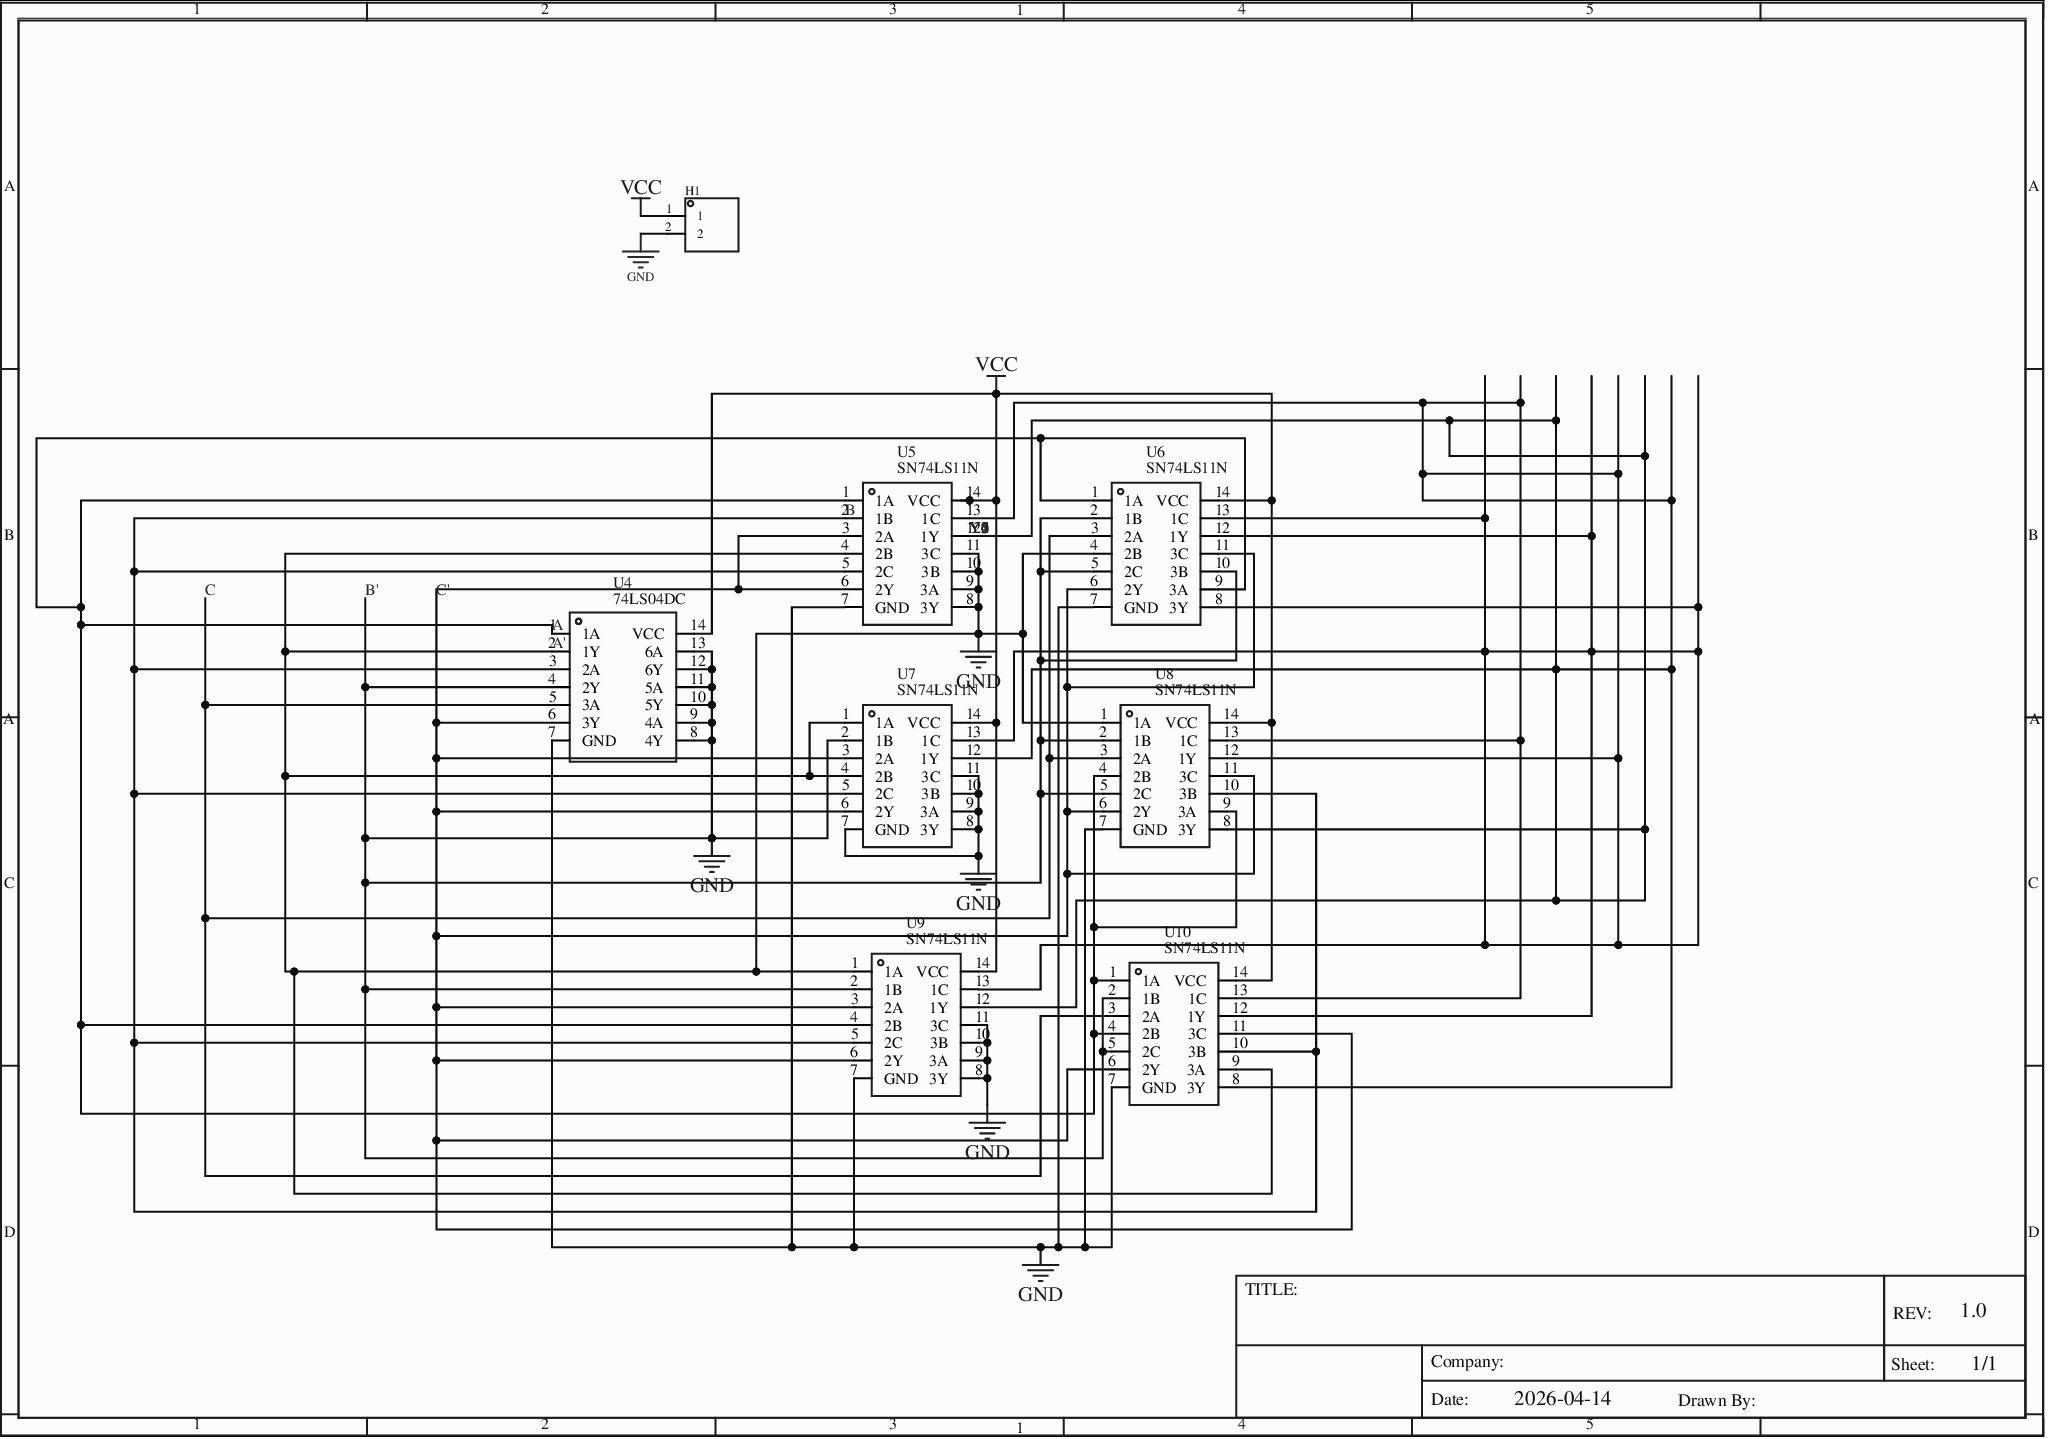
[diagram p0: MISC52068-3.schdoc]
# Altium project MISC52068-2.PrjPcb
3 sheets, 29 parts. Net scope: global (net labels, ports and power ports of the same name join across sheets).
Board file: MISC52068.pcbdoc
Sheets:
  MISC52068-3.schdoc
  MISC52068-4.schdoc
  MISC52068-5.schdoc

## Sheet MISC52068-3.schdoc
size 292 x 205 mm; Name: MISC52068; @Project Name: MISC52068; REV: 1.0; Date: 2026-04-14; Sheet: 1/1; Manufacturer Part: ?

### Parts
H1  (no value)  [HDR-TH_2P-P2.54-V-M-1]
U4  74LS04DC  [CDIP-14_L20.0-W6.8-P2.54-LS7.8-BL]
U5  SN74LS11N  [PDIP-14_L19.3-W6.4-P2.54-LS7.9-BL-1]
U6  SN74LS11N  [PDIP-14_L19.3-W6.4-P2.54-LS7.9-BL-1]
U7  SN74LS11N  [PDIP-14_L19.3-W6.4-P2.54-LS7.9-BL-1]
U8  SN74LS11N  [PDIP-14_L19.3-W6.4-P2.54-LS7.9-BL-1]
U9  SN74LS11N  [PDIP-14_L19.3-W6.4-P2.54-LS7.9-BL-1]
U10  SN74LS11N  [PDIP-14_L19.3-W6.4-P2.54-LS7.9-BL-1]

### Nets
A': H1.2 U4.2(1Y) U4.4(2Y) U4.7(GND) U4.8(4Y) U4.9(4A) U4.10(5Y) U4.11(5A) U4.12(6Y) U4.13(6A) U5.4(2B) U5.7(GND) U5.8(3Y) U5.9(3A) U5.10(3B) U5.11(3C) U6.2(1B) U6.4(2B) U6.5(2C) U6.7(GND) U6.10(3B) U7.1(1A) U7.2(1B) U7.4(2B) U7.7(GND) U7.8(3Y) U7.9(3A) U7.10(3B) U7.11(3C) U8.1(1A) U8.2(1B) U8.5(2C) U8.7(GND) U9.1(1A) U9.2(1B) U9.7(GND) U9.8(3Y) U9.9(3A) U9.10(3B) U9.11(3C) U10.2(1B) U10.5(2C) U10.7(GND) U10.9(3A)  [also labelled B', GND]
VCC: H1.1 U4.14(VCC) U5.14(VCC) U6.14(VCC) U7.14(VCC) U8.14(VCC) U9.14(VCC) U10.14(VCC)
A: U4.1(1A) U5.1(1A) U6.1(1A) U6.9(3A) U8.4(2B) U8.9(3A) U9.4(2B) U10.1(1A) U10.4(2B)
B: U4.3(2A) U5.2(1B) U5.5(2C) U7.5(2C) U8.10(3B) U9.5(2C) U10.10(3B)
C: U4.5(3A) U6.3(2A) U8.3(2A) U10.3(2A)
C': U4.6(3Y) U5.3(2A) U5.6(2Y) U6.6(2Y) U6.11(3C) U7.3(2A) U7.6(2Y) U8.6(2Y) U8.11(3C) U9.3(2A) U9.6(2Y) U10.6(2Y) U10.11(3C)
Y0: U5.12(1Y) U5.13(1C) U6.8(3Y) U6.12(1Y) U6.13(1C) U7.12(1Y) U7.13(1C) U8.8(3Y) U8.12(1Y) U8.13(1C) U9.12(1Y) U9.13(1C) U10.8(3Y) U10.12(1Y) U10.13(1C)  [also labelled Y1, Y2, Y3, Y4, Y5, Y6, Y7]

### Notes on the sheet
- 1
- 2
- 3
- 4
- 5
- A
- B
- C
- D
- TITLE:
- Company:
- Sheet:
- REV:
- 1.0
- 1/1
- Date:
- 2026-04-14
- Drawn By:

### Library data of the parts
H1 = HDR-M_2.54_1x2P: Symbol: 210S-1*2P L=11.6MMGold-plated black; ConvertToPcb: yes; ModelId: 79b2e9f2d70a4d68a1b7098f27c6d4c50819f05c4eef4c71ace90d822a990e87; ModelName: HDR-M-2.54_1x2; ModelTransform: 200,100,0,0,0,0,0,0,-118.11; Device: HDR-M_2.54_1x2P; AddInBom: yes; SupplierPart: C124375; Supplier Footprint: 插件; FootprintName: HDR-TH_2P-P2.54-V-M-1
U4 = 74LS04DC: Manufacturer: TI(德州仪器); Convert to PCB: yes; UniqueId: gge1fc2652325d13f05; Device: 74LS04DC; Supplier: LCSC; Supplier Part: C4471729; Manufacturer Part: 74LS04DC; Add into BOM: yes; SymbolName: 74LS04DC; FootprintName: CDIP-14_L20.0-W6.8-P2.54-LS7.8-BL
U5 = SN74LS11N: Manufacturer: TI(德州仪器); Convert to PCB: yes; UniqueId: gge3e49268ee8ed4b78; ModelId: 850da569defe42bfb44bffbf61585822; Device: SN74LS11N; Supplier: LCSC; Supplier Part: C2870896; Manufacturer Part: SN74LS11N; JLCPCB Part Class: Extended Part; Add into BOM: yes; SymbolName: SN74LS11N; FootprintName: PDIP-14_L19.3-W6.4-P2.54-LS7.9-BL-1; ModelName: PDIP-14_L19.3-W6.4-P2.54-LS7.9-BL-1
U6 = SN74LS11N: Manufacturer: TI(德州仪器); Convert to PCB: yes; UniqueId: gge62c023ad5ebddd35; ModelId: 850da569defe42bfb44bffbf61585822; Device: SN74LS11N; Supplier: LCSC; Supplier Part: C2870896; Manufacturer Part: SN74LS11N; JLCPCB Part Class: Extended Part; Add into BOM: yes; SymbolName: SN74LS11N; FootprintName: PDIP-14_L19.3-W6.4-P2.54-LS7.9-BL-1; ModelName: PDIP-14_L19.3-W6.4-P2.54-LS7.9-BL-1
U7 = SN74LS11N: Manufacturer: TI(德州仪器); Convert to PCB: yes; UniqueId: ggefcd329deefd429e6; ModelId: 850da569defe42bfb44bffbf61585822; Device: SN74LS11N; Supplier: LCSC; Supplier Part: C2870896; Manufacturer Part: SN74LS11N; JLCPCB Part Class: Extended Part; Add into BOM: yes; SymbolName: SN74LS11N; FootprintName: PDIP-14_L19.3-W6.4-P2.54-LS7.9-BL-1; ModelName: PDIP-14_L19.3-W6.4-P2.54-LS7.9-BL-1
U8 = SN74LS11N: Manufacturer: TI(德州仪器); Convert to PCB: yes; UniqueId: gge78541bf1d1c55658; ModelId: 850da569defe42bfb44bffbf61585822; Device: SN74LS11N; Supplier: LCSC; Supplier Part: C2870896; Manufacturer Part: SN74LS11N; JLCPCB Part Class: Extended Part; Add into BOM: yes; SymbolName: SN74LS11N; FootprintName: PDIP-14_L19.3-W6.4-P2.54-LS7.9-BL-1; ModelName: PDIP-14_L19.3-W6.4-P2.54-LS7.9-BL-1
U9 = SN74LS11N: Manufacturer: TI(德州仪器); Convert to PCB: yes; UniqueId: gge5f36f0d363a67215; ModelId: 850da569defe42bfb44bffbf61585822; Device: SN74LS11N; Supplier: LCSC; Supplier Part: C2870896; Manufacturer Part: SN74LS11N; JLCPCB Part Class: Extended Part; Add into BOM: yes; SymbolName: SN74LS11N; FootprintName: PDIP-14_L19.3-W6.4-P2.54-LS7.9-BL-1; ModelName: PDIP-14_L19.3-W6.4-P2.54-LS7.9-BL-1
U10 = SN74LS11N: Manufacturer: TI(德州仪器); Convert to PCB: yes; UniqueId: ggec3b506dc92581c8d; ModelId: 850da569defe42bfb44bffbf61585822; Device: SN74LS11N; Supplier: LCSC; Supplier Part: C2870896; Manufacturer Part: SN74LS11N; JLCPCB Part Class: Extended Part; Add into BOM: yes; SymbolName: SN74LS11N; FootprintName: PDIP-14_L19.3-W6.4-P2.54-LS7.9-BL-1; ModelName: PDIP-14_L19.3-W6.4-P2.54-LS7.9-BL-1

## Sheet MISC52068-4.schdoc
size 292 x 205 mm; Name: MISC52068; @Project Name: MISC52068; REV: 1.0; Date: 2026-04-15; Sheet: 1/1; Manufacturer Part: ?
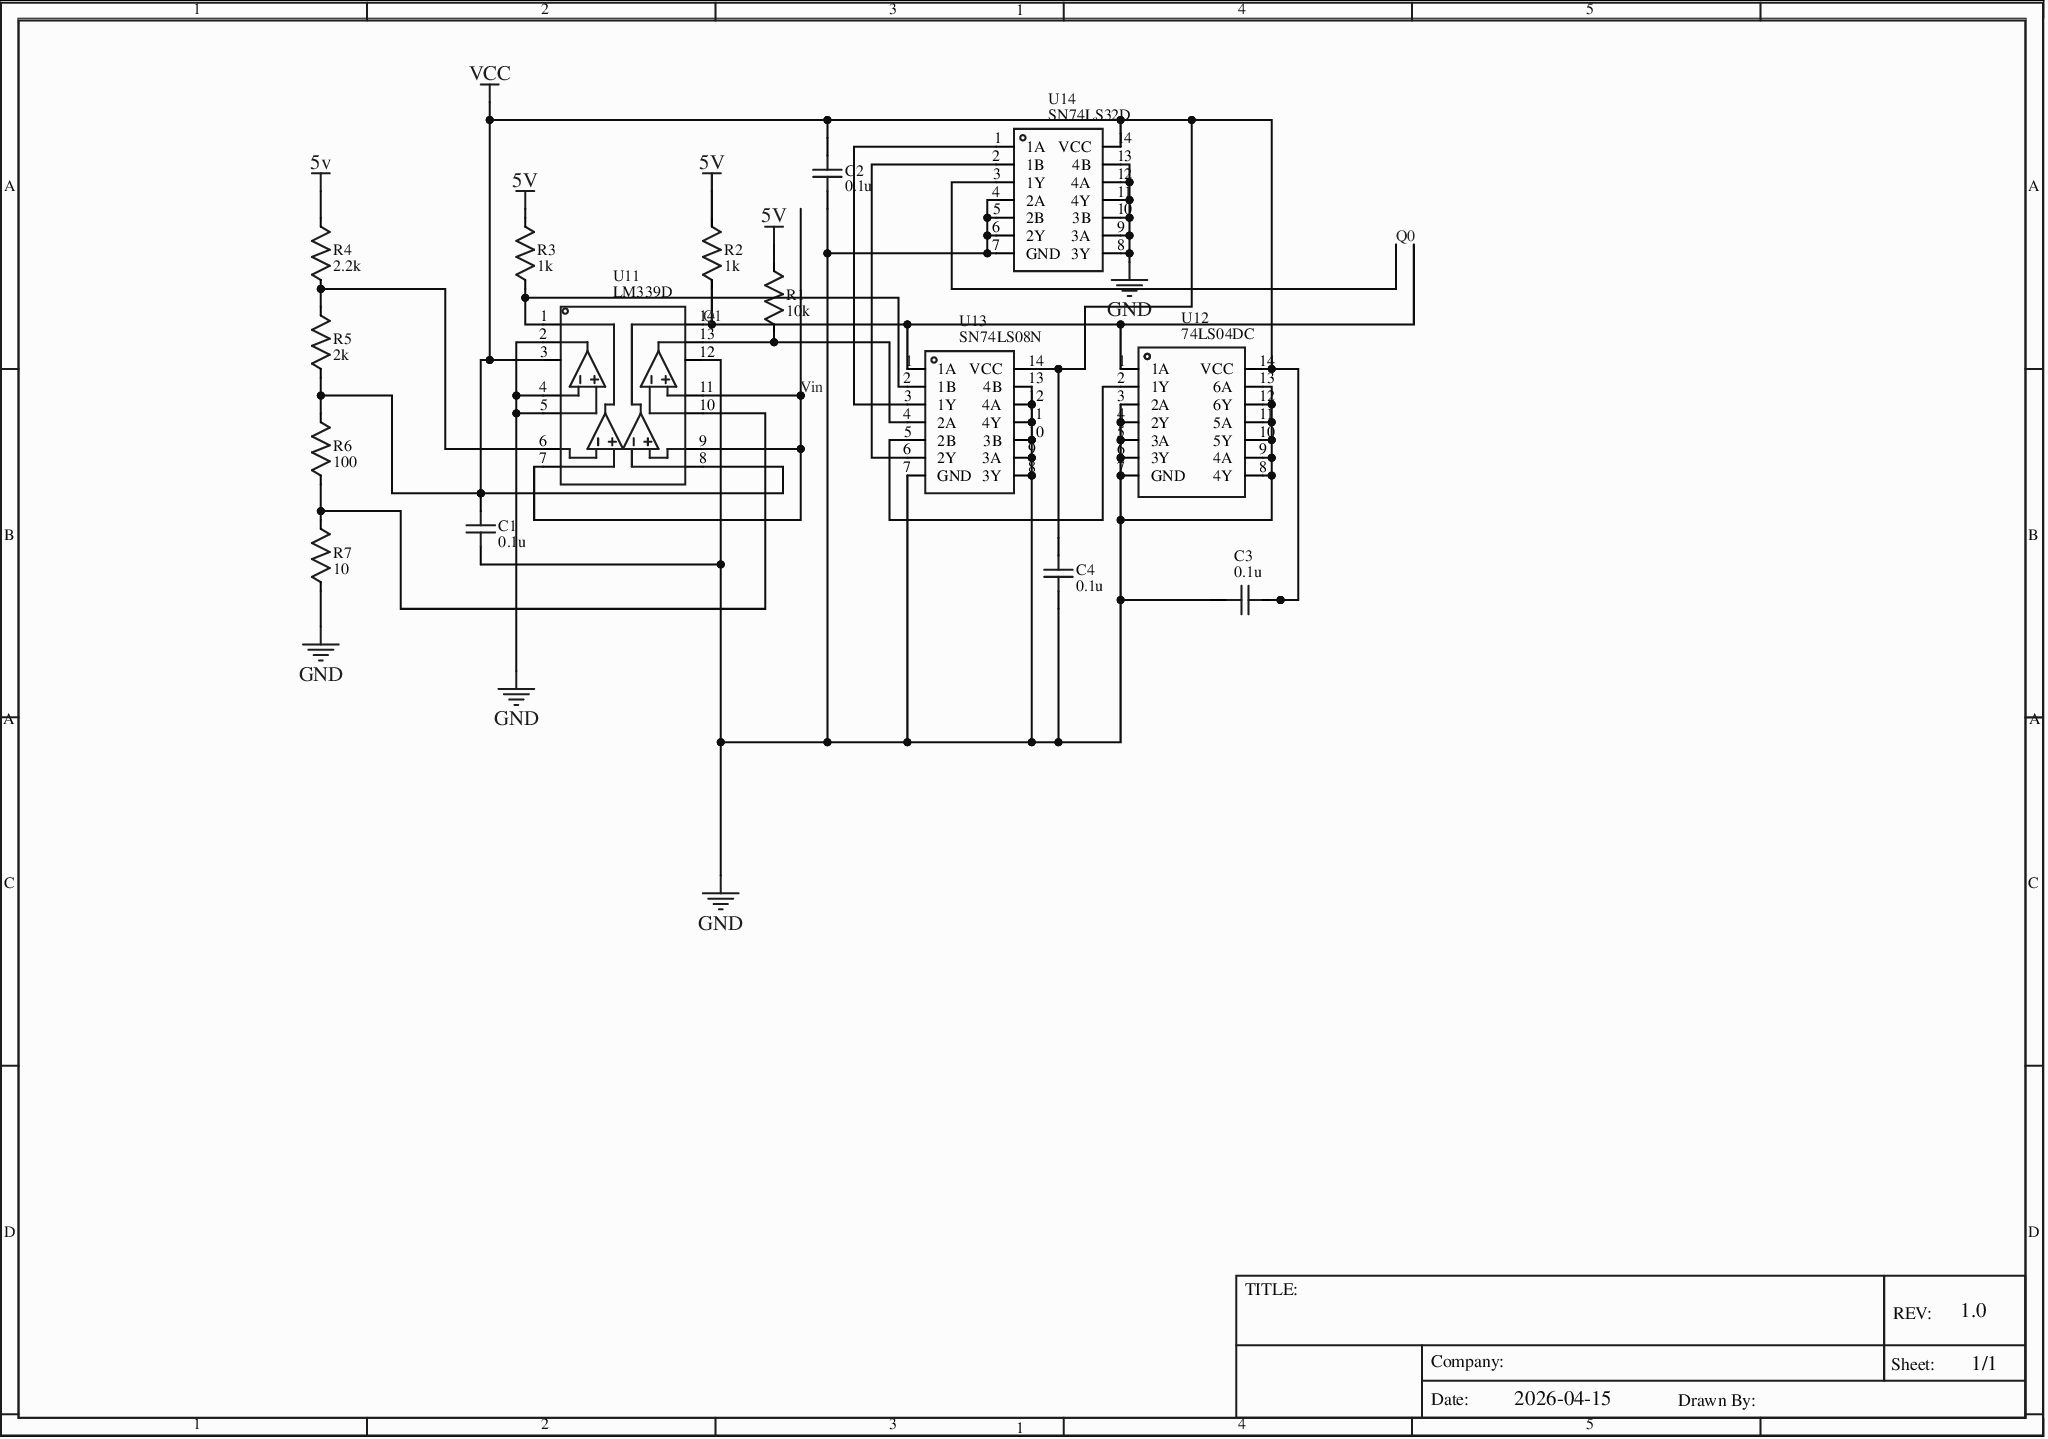
[diagram p1: MISC52068-4.schdoc]

### Parts
C1  0.1u  [C0603]
C2  0.1u  [C0603]
C3  0.1u  [C0603]
C4  0.1u  [C0603]
R1  10k  [R0603]
R2  1k  [R0603]
R3  1k  [R0603]
R4  2.2k  [R0603]
R5  2k  [R0603]
R6  100  [R0603]
R7  10  [R0603]
U11  LM339D  [SOIC-14_L8.7-W3.9-P1.27-LS6.0-BL]
U12  74LS04DC  [CDIP-14_L20.0-W6.8-P2.54-LS7.8-BL]
U13  SN74LS08N  [PDIP-14_L19.3-W6.4-P2.54-LS7.9-BL-1]
U14  SN74LS32D  [SOIC-14_L8.7-W3.9-P1.27-LS6.0-BL]

### Nets
5V: R1.1 R2.2 R3.2 R4.2
GND: C1.1 C2.1 C3.1 C4.1 R7.1 U11.2 U11.4 U11.5 U11.12(GND) U12.3(2A) U12.4(2Y) U12.5(3A) U12.6(3Y) U12.7(GND) U12.8(4Y) U12.9(4A) U12.10(5Y) U12.11(5A) U12.12(6Y) U12.13(6A) U13.7(GND) U13.8(3Y) U13.9(3A) U13.10(3B) U13.11(4Y) U13.12(4A) U13.13(4B) U14.4(2A) U14.5(2B) U14.6(2Y) U14.7(GND) U14.8(3Y) U14.9(3A) U14.10(3B) U14.11(4Y) U14.12(4A) U14.13(4B)  [project net A']
VCC: C1.2 C2.2 C3.2 C4.2 R5.1 R6.2 U11.3(VDD) U11.8 U12.14(VCC) U13.14(VCC) U14.14(VCC)
Q0: U14.3(1Y)
Q1: R2.1 U11.14 U12.1(1A) U13.1(1A)
Vin: U11.7 U11.9 U11.11
NetR1_2: R1.2 U11.13 U13.4(2A)
NetR3_1: R3.1 U11.1 U13.2(1B)
NetR4_1: R4.1 R5.2 U11.6
NetR6_1: R6.1 R7.2 U11.10
NetU12_2: U12.2(1Y) U13.5(2B)
NetU13_3: U13.3(1Y) U14.1(1A)
NetU13_6: U13.6(2Y) U14.2(1B)

### Notes on the sheet
- 1
- 2
- 3
- 4
- 5
- A
- B
- C
- D
- TITLE:
- Company:
- Sheet:
- REV:
- 1.0
- 1/1
- Date:
- 2026-04-15
- Drawn By:

### Library data of the parts
C1 = 0.1u: Convert to PCB: yes; UniqueId: gge9b4b7d5ae77fed66; ModelId: fca5be93b99f4b5a9a2fd372d58c31d9; Device: 0.1u; Add into BOM: yes; SymbolName: 0.1u; FootprintName: C0603; ModelName: C0603
C2 = 0.1u: Convert to PCB: yes; UniqueId: gge91caf2415d14d8a6; ModelId: fca5be93b99f4b5a9a2fd372d58c31d9; Device: 0.1u; Add into BOM: yes; SymbolName: 0.1u; FootprintName: C0603; ModelName: C0603
C3 = 0.1u: Convert to PCB: yes; UniqueId: gge059f44ceb39db7ba; ModelId: fca5be93b99f4b5a9a2fd372d58c31d9; Device: 0.1u; Add into BOM: yes; SymbolName: 0.1u; FootprintName: C0603; ModelName: C0603
C4 = 0.1u: Convert to PCB: yes; UniqueId: ggebd1fa56daf418cba; ModelId: fca5be93b99f4b5a9a2fd372d58c31d9; Device: 0.1u; Add into BOM: yes; SymbolName: 0.1u; FootprintName: C0603; ModelName: C0603
R1 = 10k: Convert to PCB: yes; UniqueId: gge2970eafe3c3c4cd1; ModelId: fc143cca1e79419f9cd78b61e9279f08; Device: 10k; Add into BOM: yes; SymbolName: 10k; FootprintName: R0603; ModelName: R0603
R2 = 1k: Convert to PCB: yes; UniqueId: gge7a1a84ea6c144b07; ModelId: fc143cca1e79419f9cd78b61e9279f08; Device: 1k; Add into BOM: yes; SymbolName: 1k; FootprintName: R0603; ModelName: R0603
R3 = 1k: Convert to PCB: yes; UniqueId: gge524ddc4880260f4a; ModelId: fc143cca1e79419f9cd78b61e9279f08; Device: 1k; Add into BOM: yes; SymbolName: 1k; FootprintName: R0603; ModelName: R0603
R4 = 2.2k: Convert to PCB: yes; UniqueId: ggea6b97da8000b69b1; ModelId: fc143cca1e79419f9cd78b61e9279f08; Device: 2.2k; Add into BOM: yes; SymbolName: 2.2k; FootprintName: R0603; ModelName: R0603
R5 = 2k: Convert to PCB: yes; UniqueId: ggec015f059d36281e2; ModelId: fc143cca1e79419f9cd78b61e9279f08; Device: 2k; Add into BOM: yes; SymbolName: 2k; FootprintName: R0603; ModelName: R0603
R6 = 100: Convert to PCB: yes; UniqueId: gge93323ad735862b4e; ModelId: fc143cca1e79419f9cd78b61e9279f08; Device: 100; Add into BOM: yes; SymbolName: 100; FootprintName: R0603; ModelName: R0603
R7 = 10: Convert to PCB: yes; UniqueId: ggefc4a139e63da2681; ModelId: fc143cca1e79419f9cd78b61e9279f08; Device: 10; Add into BOM: yes; SymbolName: 10; FootprintName: R0603; ModelName: R0603
U11 = LM339D: Manufacturer: TI(德州仪器); Convert to PCB: yes; UniqueId: gge39a07b4e136ac54f; Device: LM339D; Supplier: LCSC; Supplier Part: C350549; Manufacturer Part: LM339D; JLCPCB Part Class: Extended Part; Add into BOM: yes; SymbolName: LM339D; FootprintName: SOIC-14_L8.7-W3.9-P1.27-LS6.0-BL
U12 = 74LS04DC: Manufacturer: TI(德州仪器); Convert to PCB: yes; UniqueId: gge7b3de65d559673b6; Device: 74LS04DC; Supplier: LCSC; Supplier Part: C4471729; Manufacturer Part: 74LS04DC; Add into BOM: yes; SymbolName: 74LS04DC; FootprintName: CDIP-14_L20.0-W6.8-P2.54-LS7.8-BL
U13 = SN74LS08N: Manufacturer: TI(德州仪器); Convert to PCB: yes; UniqueId: gge3a2c9d595387f8ef; ModelId: 850da569defe42bfb44bffbf61585822; Device: SN74LS08N; Supplier: LCSC; Supplier Part: C2869595; Manufacturer Part: SN74LS08N; JLCPCB Part Class: Extended Part; Add into BOM: yes; SymbolName: SN74LS08N; FootprintName: PDIP-14_L19.3-W6.4-P2.54-LS7.9-BL-1; ModelName: PDIP-14_L19.3-W6.4-P2.54-LS7.9-BL-1
U14 = SN74LS32D: Manufacturer: TI(德州仪器); Convert to PCB: yes; UniqueId: gge838f6af392a07ce1; Device: SN74LS32D; Supplier: LCSC; Supplier Part: C2869302; Manufacturer Part: SN74LS32D; JLCPCB Part Class: Extended Part; Add into BOM: yes; SymbolName: SN74LS32D; FootprintName: SOIC-14_L8.7-W3.9-P1.27-LS6.0-BL

## Sheet MISC52068-5.schdoc
size 292 x 205 mm; Name: MISC52068; @Project Name: MISC52068; REV: 1.0; Date: 2026-04-16; Sheet: 1/1; Manufacturer Part: ?
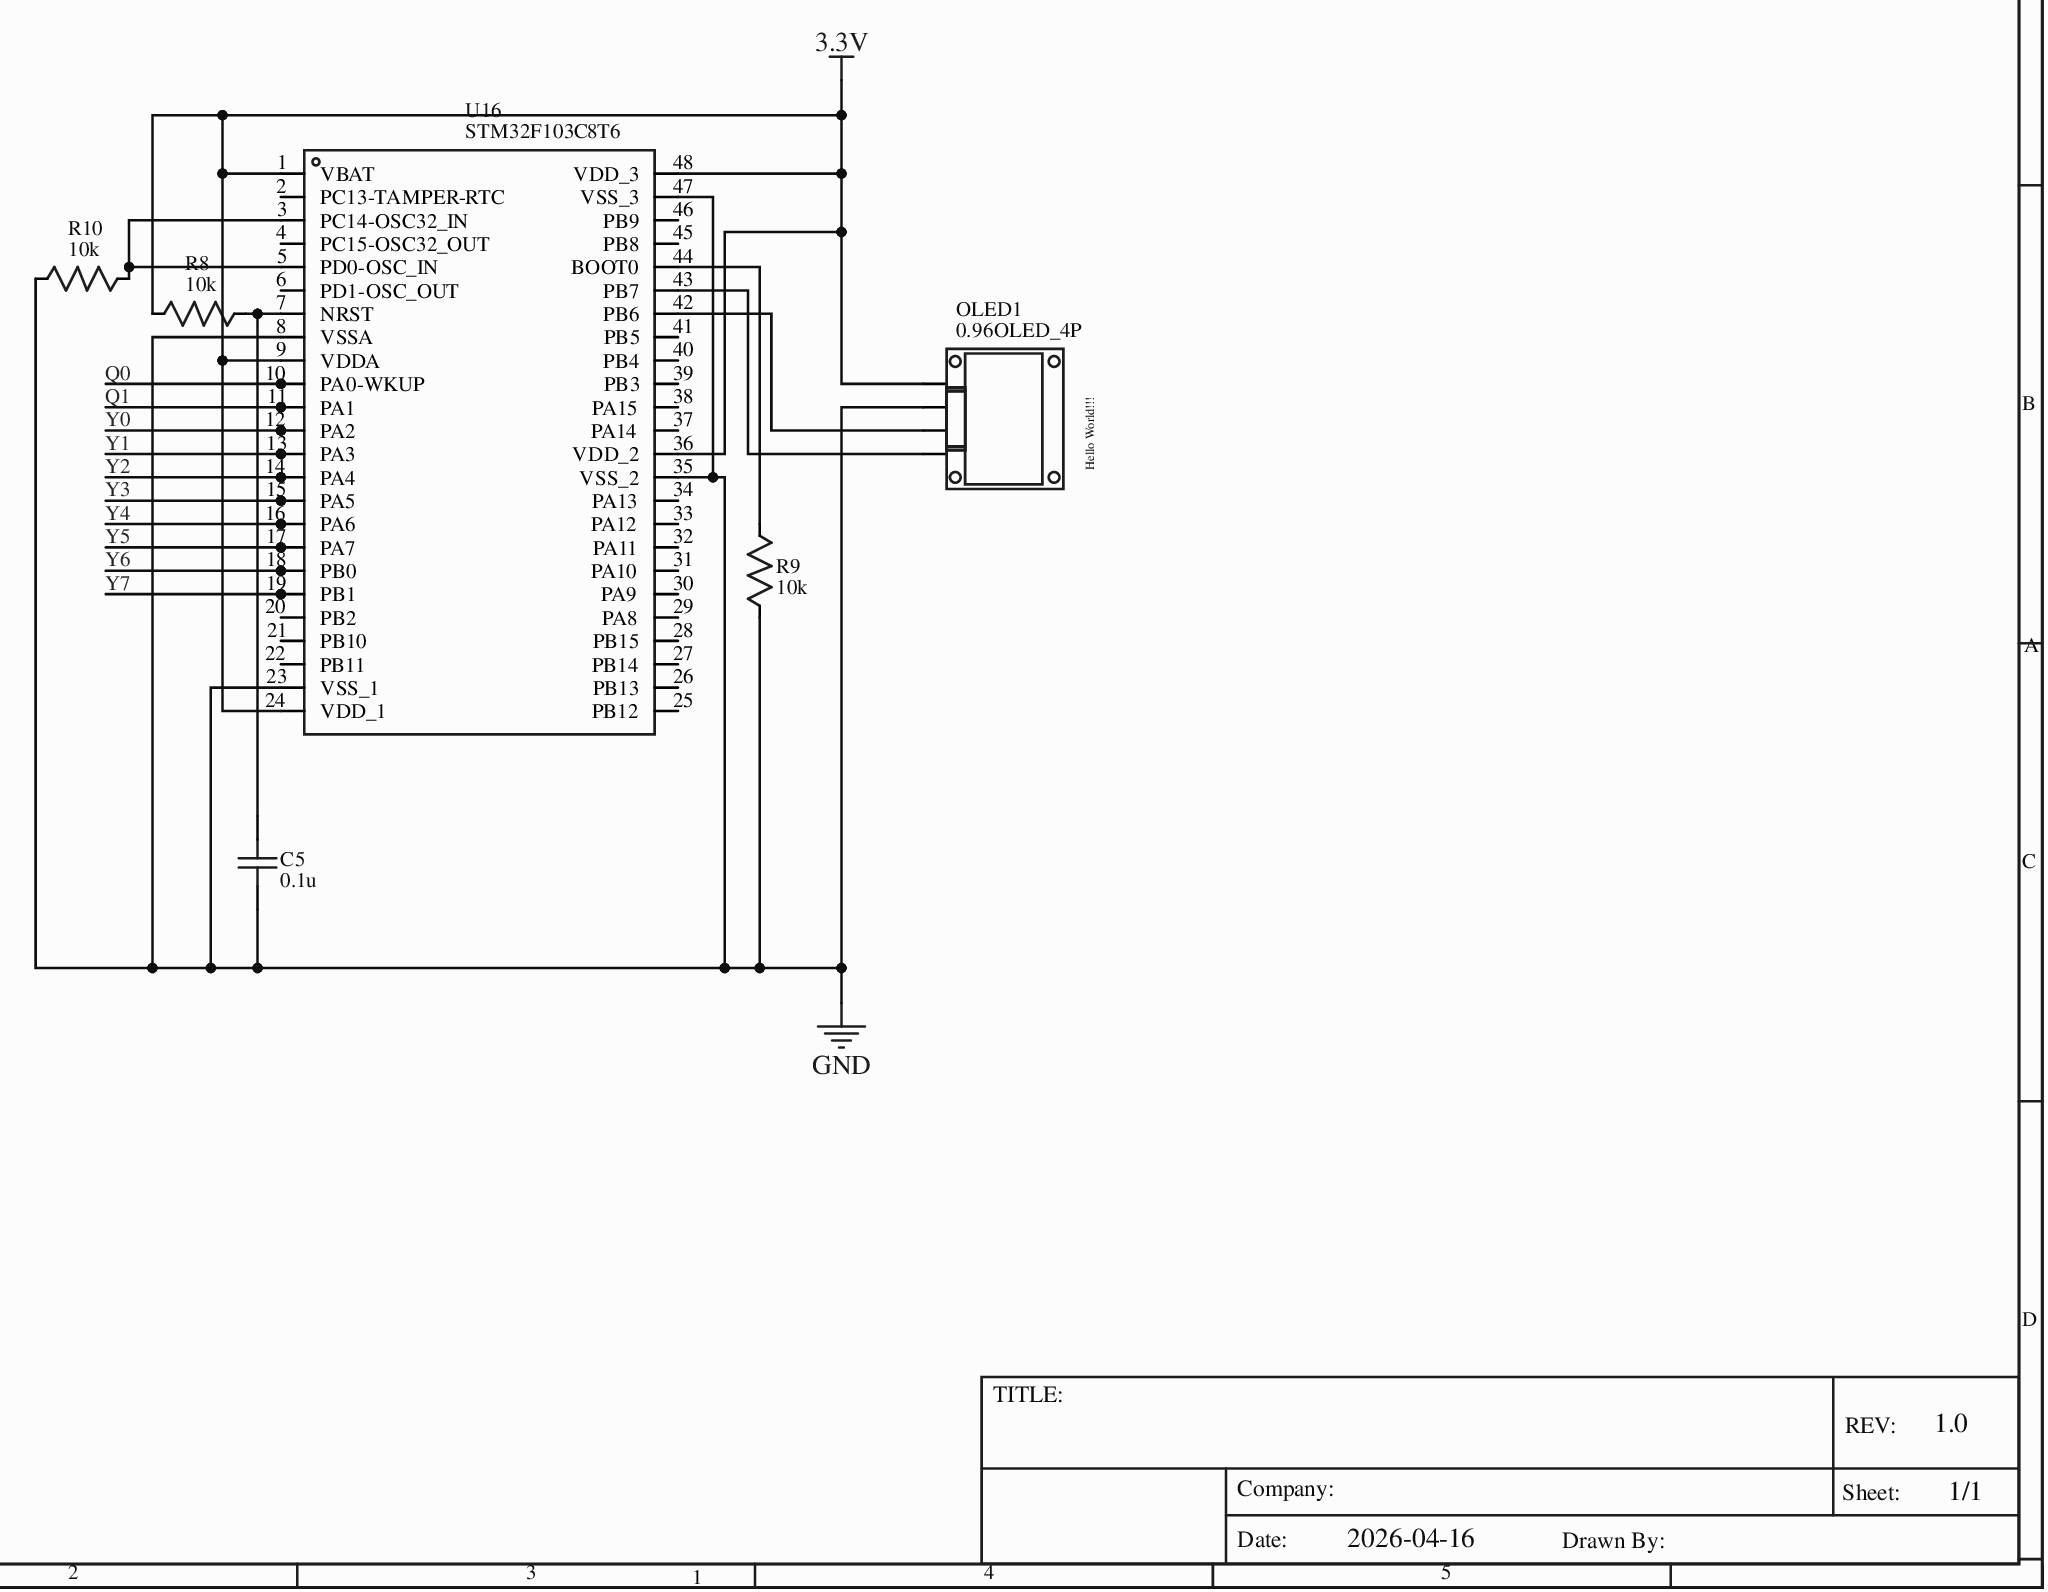
[diagram p2: MISC52068-5.schdoc]

### Parts
C5  0.1u  [C0603]
OLED1  0.96OLED_4P  [0.96OLED_4P]
R8  10k  [R0603]
R9  10k  [R0603]
R10  10k  [R0603]
U16  STM32F103C8T6  [LQFP-48_L7.0-W7.0-P0.50-LS9.0-BL]

### Nets
3.3V: OLED1.1 R8.1 U16.1(VBAT) U16.9(VDDA) U16.24(VDD_1) U16.36(VDD_2) U16.48(VDD_3)
GND: C5.1 OLED1.2 R9.1 R10.1 U16.8(VSSA) U16.23(VSS_1) U16.35(VSS_2) U16.47(VSS_3)  [project net A']
Q0: U16.10(PA0-WKUP)
Q1: U16.11(PA1)
Y0: U16.12(PA2) U16.13(PA3) U16.14(PA4) U16.15(PA5) U16.16(PA6) U16.17(PA7) U16.18(PB0) U16.19(PB1)  [also labelled Y1, Y2, Y3, Y4, Y5, Y6, Y7]
NetC5_2: C5.2 R8.2 U16.7(NRST)
NetOLED1_3: OLED1.3 U16.42(PB6)
NetOLED1_4: OLED1.4 U16.43(PB7)
NetR9_2: R9.2 U16.44(BOOT0)
NetR10_2: R10.2 U16.3(PC14-OSC32_IN) U16.5(PD0-OSC_IN)

Not connected (* = marked no-connect by the designer): U16 2(PC13-TAMPER-RTC) 4(PC15-OSC32_OUT) 6(PD1-OSC_OUT) 20(PB2) 21(PB10) 22(PB11) 25(PB12) 26(PB13) 27(PB14) 28(PB15) 29(PA8) 30(PA9) 31(PA10) 32(PA11) 33(PA12) 34(PA13) 37(PA14) 38(PA15) 39(PB3) 40(PB4) 41(PB5) 45(PB8) 46(PB9)

### Notes on the sheet
- 1
- 2
- 3
- 4
- 5
- A
- B
- C
- D
- TITLE:
- Company:
- Sheet:
- REV:
- 1.0
- 1/1
- Date:
- 2026-04-16
- Drawn By:

### Library data of the parts
C5 = 0.1u: Convert to PCB: yes; UniqueId: gge42f1ca1a3c144898; ModelId: fca5be93b99f4b5a9a2fd372d58c31d9; Device: 0.1u; Add into BOM: yes; SymbolName: 0.1u; FootprintName: C0603; ModelName: C0603
OLED1 = 0.96OLED_4P: Convert to PCB: yes; UniqueId: ggeb6856457ce4f1913; ModelId: 79c000fdb68d45a296c2e9bedf4f9055; Device: 0.96OLED_4P; Supplier: LCSC; Add into BOM: yes; SymbolName: 0.96OLED_4P; FootprintName: 0.96OLED_4P; ModelName: 0.96OLED_4P
R8 = 10k: Convert to PCB: yes; UniqueId: gge6d97d05386875263; ModelId: fc143cca1e79419f9cd78b61e9279f08; Device: 10k; Add into BOM: yes; SymbolName: 10k; FootprintName: R0603; ModelName: R0603
R9 = 10k: Convert to PCB: yes; UniqueId: gge5a39fe30ebb05b17; ModelId: fc143cca1e79419f9cd78b61e9279f08; Device: 10k; Add into BOM: yes; SymbolName: 10k; FootprintName: R0603; ModelName: R0603
R10 = 10k: Convert to PCB: yes; UniqueId: gge2a6448e050eddb72; ModelId: fc143cca1e79419f9cd78b61e9279f08; Device: 10k; Add into BOM: yes; SymbolName: 10k; FootprintName: R0603; ModelName: R0603
U16 = STM32F103C8T6: Manufacturer: ST(意法半导体); Convert to PCB: yes; UniqueId: gge20ee08fc12a282d6; Device: STM32F103C8T6; Supplier: LCSC; Manufacturer Part: STM32F103C8T6; Supplier Part: C8734; JLCPCB Part Class: Extended Part; Add into BOM: yes; SymbolName: STM32F103C8T6; FootprintName: LQFP-48_L7.0-W7.0-P0.50-LS9.0-BL

## Nets that join several sheets
A': MISC52068-3 (44 pins), MISC52068-4 (37 pins), MISC52068-5 (8 pins)
VCC: MISC52068-3 (8 pins), MISC52068-4 (11 pins)
Q0: MISC52068-4 (U14.3), MISC52068-5 (U16.10)
Q1: MISC52068-4 (R2.1 U11.14 U12.1 U13.1), MISC52068-5 (U16.11)
Y0: MISC52068-3 (15 pins), MISC52068-5 (8 pins)